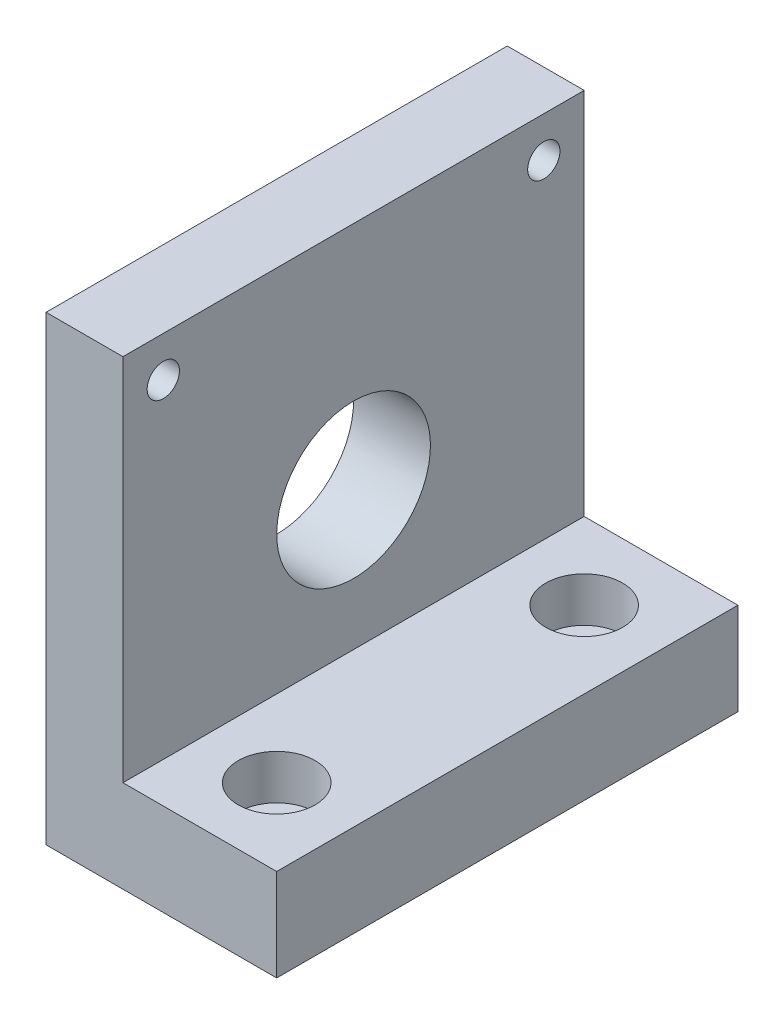
SolidWorks part; units mm, degrees
ref_plane "前视基准面" through (0, 0, 0) normal (0, 0, 1) x (1, 0, 0)
ref_plane "上视基准面" through (0, 0, 0) normal (0, 1, 0) x (1, 0, 0)
ref_plane "右视基准面" through (0, 0, 0) normal (1, 0, 0) x (0, 0, -1)
sketch "草图1" plane through (0, 0, 0) normal (0, 0, 1) x (1, 0, 0)
  line L0 (-12.8923, 45.3231) -> (-12.8923, -2.6769)
  line L1 (-12.8923, -2.6769) -> (7.1077, -2.6769)
  line L2 (7.1077, -2.6769) -> (7.1077, -14.6769)
  line L3 (7.1077, -14.6769) -> (-22.8923, -14.6769)
  line L4 (-22.8923, -14.6769) -> (-22.8923, 45.3231)
  line L5 (-22.8923, 45.3231) -> (-12.8923, 45.3231)
  dimension "D1" = 12
  dimension "D2" = 30
  dimension "D3" = 10
  dimension "D4" = 60
extrude "凸台-拉伸1" add sketch "草图1" along normal blind 60
sketch "草图2" plane through (-12.8923, 0, 0) normal (1, 0, 0) x (0, 0, -1)
  line L0 (-60, 45.3231) -> (0, 45.3231) construction
  line L1 (-60, -2.6769) -> (-60, 45.3231) construction
  circle A0 centre (-30, 15.3231) radius 10
  dimension "D1" = 20
  dimension "D2" = 30
  dimension "D3" = 30
extrude "切除-拉伸1" cut sketch "草图2" against normal through all
sketch "草图3" plane through (-12.8923, 0, 0) normal (1, 0, 0) x (0, 0, -1)
  line L0 (-60, 45.3231) -> (0, 45.3231) construction
  line L1 (-60, -2.6769) -> (-60, 45.3231) construction
  line L2 (0, -2.6769) -> (0, 45.3231) construction
  circle A0 centre (-54.75, 40.0731) radius 2.1
  circle A1 centre (-5.25, 40.0731) radius 2.1
  dimension "D1" = 4.2
  dimension "D4" = 4.2
  dimension "D2" = 5.25
  dimension "D3" = 5.25
  dimension "D5" = 5.25
  dimension "D6" = 5.25
extrude "切除-拉伸2" cut sketch "草图3" against normal through all
sketch "草图4" plane through (0, -2.6769, 0) normal (0, 1, 0) x (1, 0, 0)
  line L0 (7.1077, -60) -> (7.1077, 0) construction
  line L1 (7.1077, -60) -> (-12.8923, -60) construction
  line L2 (7.1077, 0) -> (-12.8923, 0) construction
  circle A0 centre (-2.8923, -10) radius 2.75
  circle A1 centre (-2.8923, -50) radius 2.75
  dimension "D1" = 5.5
  dimension "D2" = 5.5
  dimension "D3" = 10
  dimension "D4" = 10
  dimension "D5" = 10
  dimension "D6" = 10
extrude "切除-拉伸3" cut sketch "草图4" against normal through all
sketch "草图5" plane through (0, -2.6769, 0) normal (0, 1, 0) x (1, 0, 0)
  circle A0 centre (-2.8923, -10) radius 5
  circle A1 centre (-2.8923, -50) radius 5
  dimension "D1" = 10
  dimension "D2" = 10
extrude "切除-拉伸4" cut sketch "草图5" against normal blind 5.8
